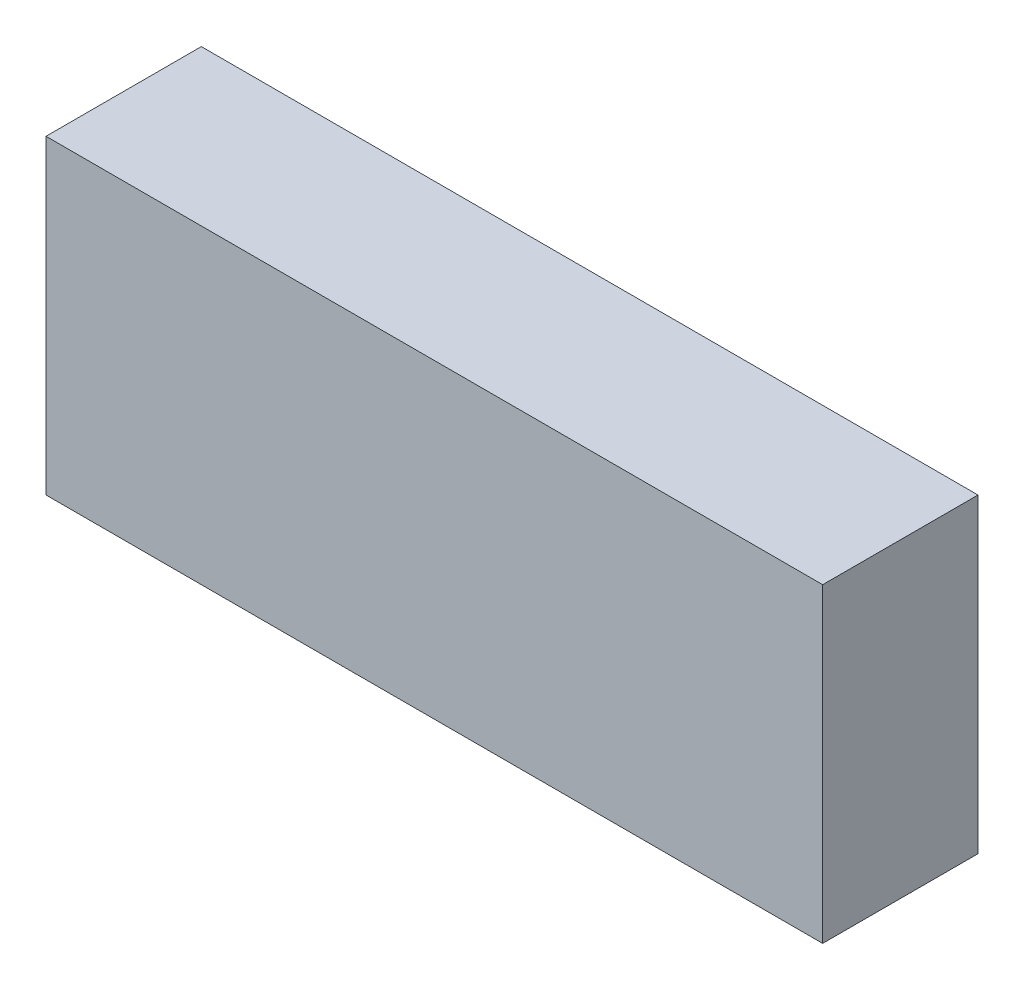
from build123d import *

# Parameters (mm, degrees)
SKETCH1_W           = 50
SKETCH1_H           = 20
BOSS_EXTRUDE1_DEPTH = 10


with BuildPart() as part:
    # Sketch1 → Boss-Extrude1 (new body)
    with BuildSketch(Plane.XY):
        Rectangle(SKETCH1_W, SKETCH1_H)
    extrude(amount=BOSS_EXTRUDE1_DEPTH)


solid = part.part
